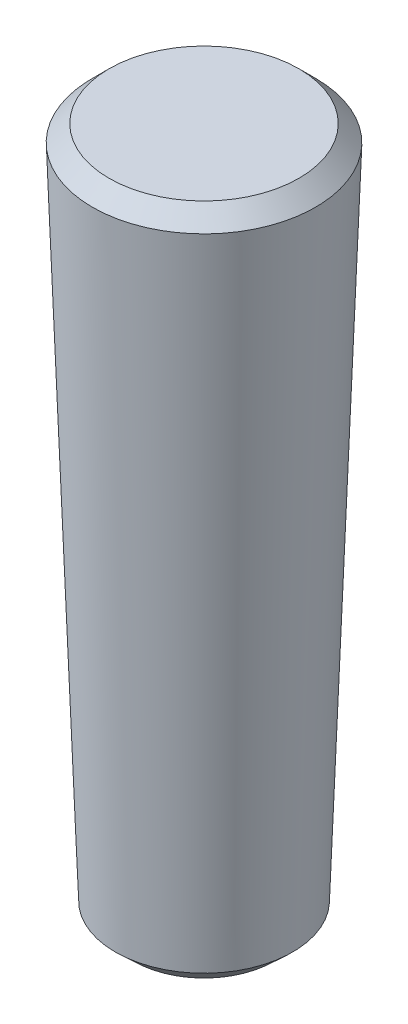
from build123d import *
from OCP.BRepFilletAPI import BRepFilletAPI_MakeChamfer

# Parameters (mm, degrees)
CHAMFER1_SIZE    = 1
CHAMFER1_SIZE2   = 1.036815955
CHAMFER1_SIZE2_2 = 0.96684652


with BuildPart() as part:
    # Sketch1 → Revolve4 (revolve)
    with BuildSketch(Plane.XY, mode=Mode.PRIVATE) as revolve4_sk:
        Polygon((6.5, 40), (5.10316922, 0), (0, 0), (0, 40), align=None)
    revolve(revolve4_sk.sketch.rotate(Axis((0, 0, 0), (0, 1, 0)), 90), axis=Axis((0, 0, 0), (0, 1, 0)))

    # Chamfer1: one chamfer whose edges measure the first distance from different faces: ONE call of the kernel's chamfer builder (chamfer() names one face for all edges)
    chamfer1_edges_1 = [part.edges().sort_by_distance(p)[0] for p in [
        (0, 0, 5.10316922),
    ]]
    chamfer1_side_1 = [part.faces().sort_by_distance(p)[0] for p in [
        (0, 20, 5.80158461),
    ]]
    chamfer1_edges_2 = [part.edges().sort_by_distance(p)[0] for p in [
        (0, 40, 6.5),
    ]]
    chamfer1_side_2 = [part.faces().sort_by_distance(p)[0] for p in [
        (0, 40, 0),
    ]]
    chamfer1 = BRepFilletAPI_MakeChamfer(part.part.solid().wrapped)
    for e in chamfer1_edges_1:
        chamfer1.Add(CHAMFER1_SIZE, CHAMFER1_SIZE2, e.wrapped, chamfer1_side_1[0].wrapped)  # the first distance lies on this face
    for e in chamfer1_edges_2:
        chamfer1.Add(CHAMFER1_SIZE, CHAMFER1_SIZE2_2, e.wrapped, chamfer1_side_2[0].wrapped)  # the first distance lies on this face
    add(Compound.cast(chamfer1.Shape()), mode=Mode.REPLACE)


solid = part.part
